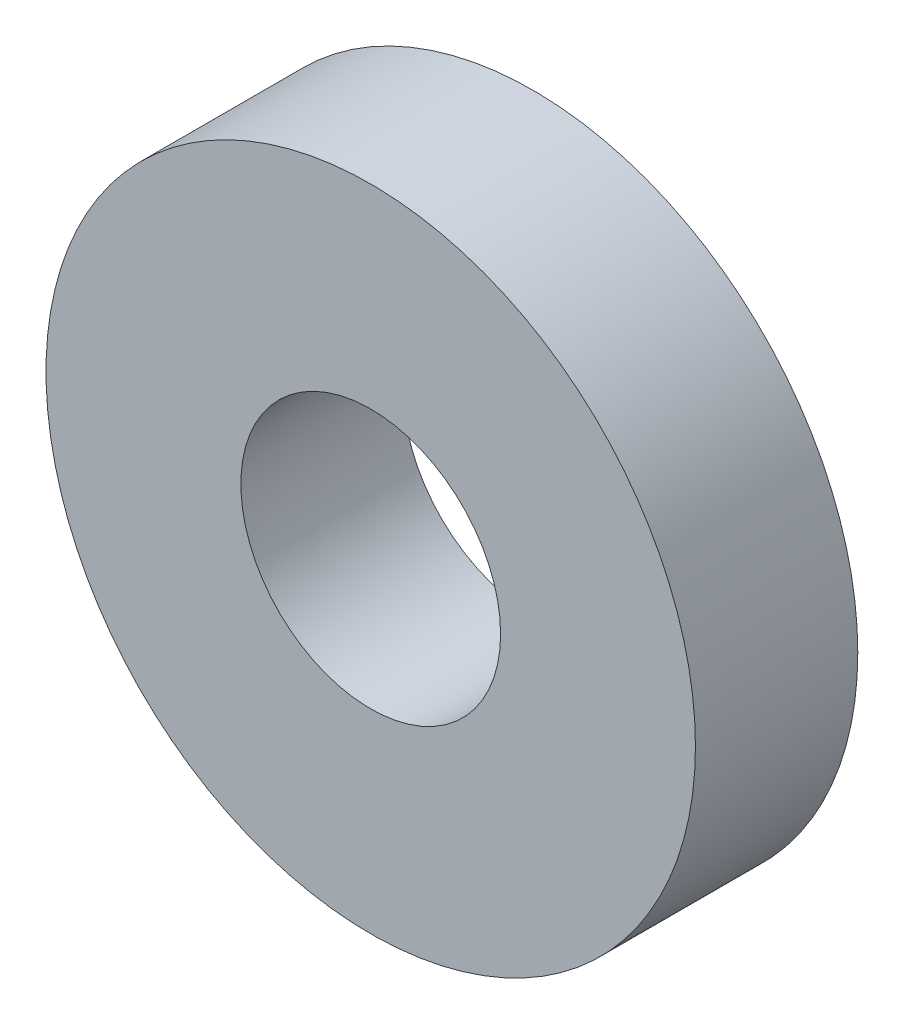
SolidWorks part; units mm, degrees
ref_plane "Front Plane" through (0, 0, 0) normal (0, 0, 1) x (1, 0, 0)
ref_plane "Top Plane" through (0, 0, 0) normal (0, 1, 0) x (1, 0, 0)
ref_plane "Right Plane" through (0, 0, 0) normal (1, 0, 0) x (0, 0, -1)
other "Configuration Table"
sketch "Sketch1" plane through (0, 0, 0) normal (0, 0, 1) x (1, 0, 0)
  circle A0 centre (0, 0) radius 4
  circle A1 centre (0, 0) radius 1.6
extrude "Boss-Extrude1" add sketch "Sketch1" along normal blind 2
